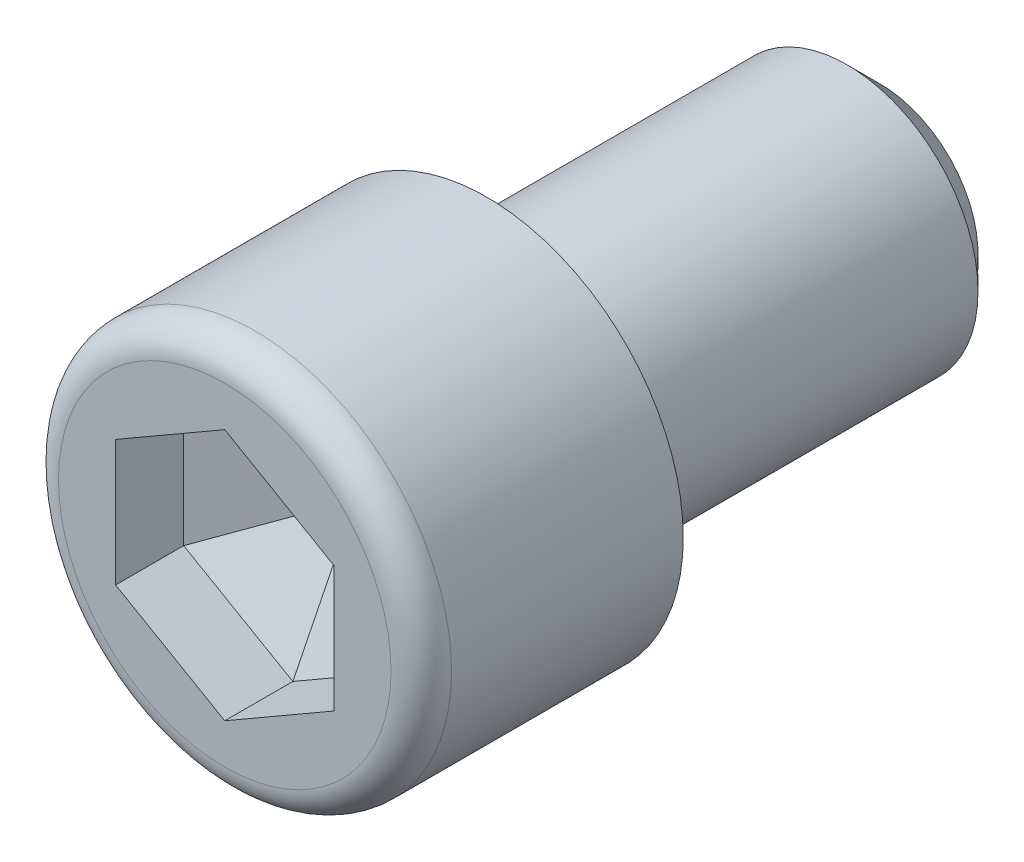
from build123d import *
from OCP.BRepFilletAPI import BRepFilletAPI_MakeChamfer

# Parameters (mm, degrees)
SKETCH1_R           = 9
BOSS_EXTRUDE1_DEPTH = 12
CUT_EXTRUDE1_DEPTH  = 6
SKETCH3_R           = 6
BOSS_EXTRUDE2_DEPTH = 18
CHAMFER1_SIZE       = 1.5
FILLET1_R           = 1.384615385
CHAMFER2_SIZE       = 2.88184438
CHAMFER2_SIZE2      = 4.991500886
FILLET2_R           = 0.1


with BuildPart() as part:
    # Sketch1 → Boss-Extrude1 (new body)
    with BuildSketch(Plane.XY):
        Circle(SKETCH1_R)
    extrude(amount=BOSS_EXTRUDE1_DEPTH)

    # Sketch2 → Cut-Extrude1 (cut)
    with BuildSketch(Plane.XY.offset(12)):
        Polygon((5, 2.886751346), (0, 5.773502692), (-5, 2.886751346), (-5, -2.886751346), (0, -5.773502692), (5, -2.886751346), align=None)
    extrude(amount=-CUT_EXTRUDE1_DEPTH, mode=Mode.SUBTRACT)

    # Sketch3 → Boss-Extrude2 (add)
    with BuildSketch(Plane(origin=(0, 0, 0), x_dir=(-1, 0, 0), z_dir=(0, 0, -1))):
        with Locations(Location((0, 0, 0), (0, 0, 180))):
            Circle(SKETCH3_R)
    extrude(amount=BOSS_EXTRUDE2_DEPTH)

    # Chamfer1
    chamfer1_edges = [part.edges().sort_by_distance(p)[0] for p in [
        (-6, 0, -18),
    ]]
    chamfer(chamfer1_edges, length=CHAMFER1_SIZE)

    # Fillet1
    fillet1_edges = [part.edges().sort_by_distance(p)[0] for p in [
        (-9, 0, 12),
    ]]
    fillet(fillet1_edges, radius=FILLET1_R)

    # Chamfer2: one chamfer whose edges measure the first distance from different faces: ONE call of the kernel's chamfer builder (chamfer() names one face for all edges)
    chamfer2_edges_1 = [part.edges().sort_by_distance(p)[0] for p in [
        (-2.5, 4.330127019, 6),
    ]]
    chamfer2_side_1 = [part.faces().sort_by_distance(p)[0] for p in [
        (-2.5, 4.330127019, 9),
    ]]
    chamfer2_edges_2 = [part.edges().sort_by_distance(p)[0] for p in [
        (2.5, 4.330127019, 6),
    ]]
    chamfer2_side_2 = [part.faces().sort_by_distance(p)[0] for p in [
        (2.5, 4.330127019, 9),
    ]]
    chamfer2_edges_3 = [part.edges().sort_by_distance(p)[0] for p in [
        (5, 0, 6),
    ]]
    chamfer2_side_3 = [part.faces().sort_by_distance(p)[0] for p in [
        (5, 0, 9),
    ]]
    chamfer2_edges_4 = [part.edges().sort_by_distance(p)[0] for p in [
        (2.5, -4.330127019, 6),
    ]]
    chamfer2_side_4 = [part.faces().sort_by_distance(p)[0] for p in [
        (2.5, -4.330127019, 9),
    ]]
    chamfer2_edges_5 = [part.edges().sort_by_distance(p)[0] for p in [
        (-2.5, -4.330127019, 6),
    ]]
    chamfer2_side_5 = [part.faces().sort_by_distance(p)[0] for p in [
        (-2.5, -4.330127019, 9),
    ]]
    chamfer2_edges_6 = [part.edges().sort_by_distance(p)[0] for p in [
        (-5, 0, 6),
    ]]
    chamfer2_side_6 = [part.faces().sort_by_distance(p)[0] for p in [
        (-5, 0, 9),
    ]]
    chamfer2 = BRepFilletAPI_MakeChamfer(part.part.solid().wrapped)
    for e in chamfer2_edges_1:
        chamfer2.Add(CHAMFER2_SIZE, CHAMFER2_SIZE2, e.wrapped, chamfer2_side_1[0].wrapped)  # the first distance lies on this face
    for e in chamfer2_edges_2:
        chamfer2.Add(CHAMFER2_SIZE, CHAMFER2_SIZE2, e.wrapped, chamfer2_side_2[0].wrapped)  # the first distance lies on this face
    for e in chamfer2_edges_3:
        chamfer2.Add(CHAMFER2_SIZE, CHAMFER2_SIZE2, e.wrapped, chamfer2_side_3[0].wrapped)  # the first distance lies on this face
    for e in chamfer2_edges_4:
        chamfer2.Add(CHAMFER2_SIZE, CHAMFER2_SIZE2, e.wrapped, chamfer2_side_4[0].wrapped)  # the first distance lies on this face
    for e in chamfer2_edges_5:
        chamfer2.Add(CHAMFER2_SIZE, CHAMFER2_SIZE2, e.wrapped, chamfer2_side_5[0].wrapped)  # the first distance lies on this face
    for e in chamfer2_edges_6:
        chamfer2.Add(CHAMFER2_SIZE, CHAMFER2_SIZE2, e.wrapped, chamfer2_side_6[0].wrapped)  # the first distance lies on this face
    add(Compound.cast(chamfer2.Shape()), mode=Mode.REPLACE)

    # Fillet2
    fillet2_edges = [part.edges().sort_by_distance(p)[0] for p in [
        (-6, 0, 0),
    ]]
    fillet(fillet2_edges, radius=FILLET2_R)


solid = part.part
